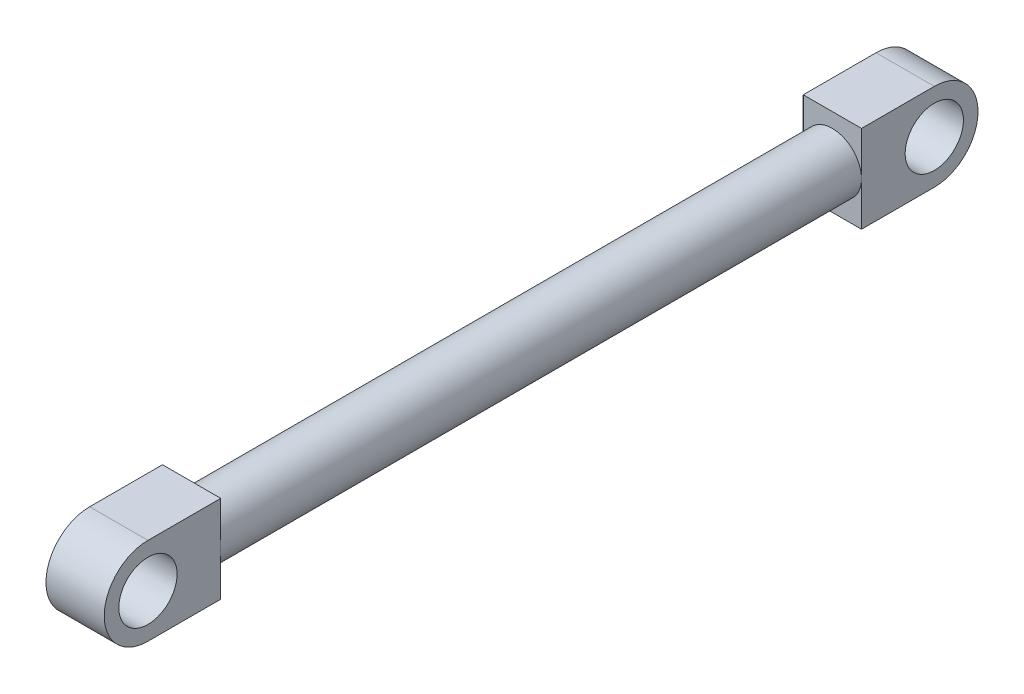
from build123d import *

# Parameters (mm, degrees)
SKETCH1_R           = 5
BOSS_EXTRUDE1_DEPTH = 110
SKETCH2_W           = 10
SKETCH2_H           = 15
BOSS_EXTRUDE2_DEPTH = 20
SKETCH3_W           = 10
SKETCH3_H           = 15
BOSS_EXTRUDE3_DEPTH = 20
SKETCH4_R           = 5
CUT_EXTRUDE1_DEPTH  = 131.599578866


with BuildPart() as part:
    # Sketch1 → Boss-Extrude1 (new body)
    with BuildSketch(Plane.XY):
        Circle(SKETCH1_R)
    extrude(amount=BOSS_EXTRUDE1_DEPTH)

    # Sketch2 → Boss-Extrude2 (add)
    with BuildSketch(Plane(origin=(0, 0, 0), x_dir=(-1, 0, 0), z_dir=(0, 0, -1))):
        Rectangle(SKETCH2_W, SKETCH2_H)
    extrude(amount=BOSS_EXTRUDE2_DEPTH)

    # Sketch3 → Boss-Extrude3 (add)
    with BuildSketch(Plane.XY.offset(110)):
        Rectangle(SKETCH3_W, SKETCH3_H)
    extrude(amount=BOSS_EXTRUDE3_DEPTH)

    # Sketch4 → Cut-Extrude1 (cut, through all)
    with BuildSketch(Plane(origin=(5, 0, 0), x_dir=(0, 0, -1), z_dir=(1, 0, 0))):
        with Locations((12.5, 0)):
            Circle(SKETCH4_R)
        with Locations((-122.5, 0)):
            Circle(SKETCH4_R)
        with BuildLine():
            Line((12.5, -7.5), (27.957175819, -19.344646022))
            Line((27.957175819, -19.344646022), (25.412525065, 11.111642689))
            Line((25.412525065, 11.111642689), (12.5, 7.5))
            ThreePointArc((12.5, 7.5), (20, 0), (12.5, -7.5))
        make_face()
        with BuildLine():
            Line((-122.5, 7.5), (-386.499272389, 23.053021062))
            Line((-386.499272389, 23.053021062), (-390.004854727, -19.344646022))
            Line((-390.004854727, -19.344646022), (-122.5, -7.5))
            ThreePointArc((-122.5, -7.5), (-130, 0), (-122.5, 7.5))
        make_face()
    extrude(amount=-CUT_EXTRUDE1_DEPTH, mode=Mode.SUBTRACT)


solid = part.part
